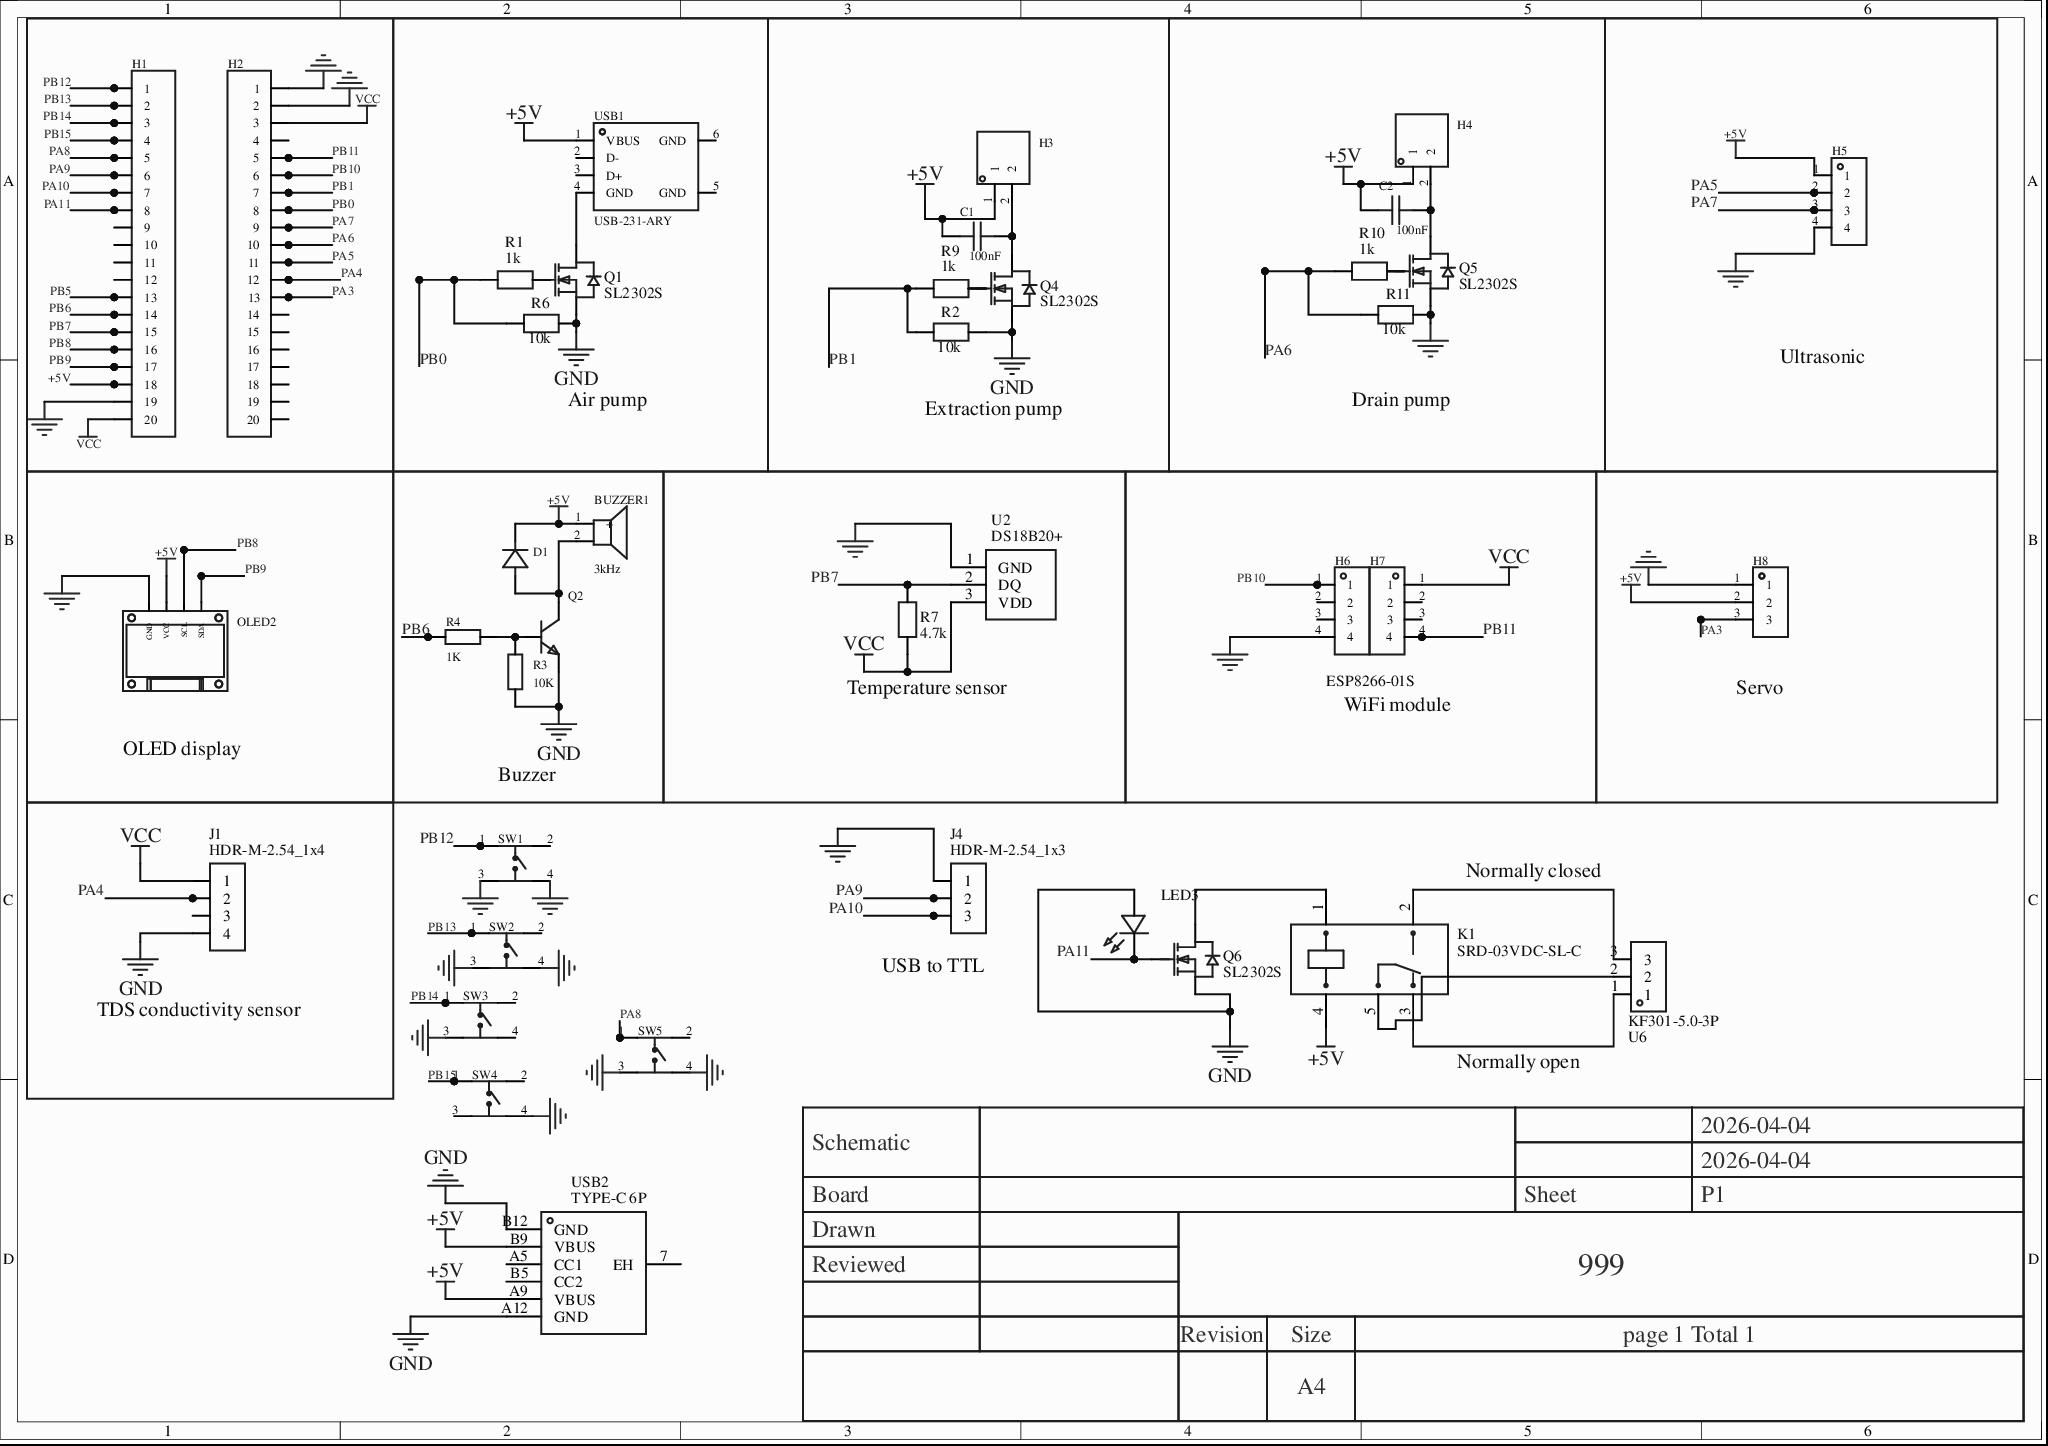
[diagram p0: MISC75408-3.schdoc]
# Altium project MISC75408-2.PrjPcb
1 sheet, 40 parts. Net scope: global (net labels, ports and power ports of the same name join across sheets).
Board file: MISC75408.pcbdoc

## Sheet MISC75408-3.schdoc
size 297 x 209 mm; Version: V1.0; @Project Name: MISC75408; @Update Date: 2026-04-16; @Create Date: 2026-04-16; @Board Name: MISC75408; @Create Time: 13:37:19; @Page Count: 1; @Page No: 1; @Schematic Name: MISC75408; @Update Time: 13:37:19; Size: A4

### Parts
BUZZER1  3kHz  [BUZ-TH_BD9.6-P5.00-D0.7-FD]
C1  100nF  [C0805]
C2  100nF  [C0805]
D1  (no value)  [DO_1N4007]
H1  (no value)  [HDR-TH_20P-P2.54-V-F]
H2  (no value)  [HDR-TH_20P-P2.54-V-F]
H3  (no value)  [HDR-TH_2P-P2.54-V-M-1]
H4  (no value)  [HDR-TH_2P-P2.54-V-M-1]
H5  (no value)  [HDR-TH_4P-P2.54-V-M]
H6  (no value)  [HDR-TH_4P-P2.54-V-M]
H7  (no value)  [HDR-TH_4P-P2.54-V-M]
H8  (no value)  [HDR-TH_3P-P2.54-V-M]
J1  HDR-M-2.54_1x4  [HDR-M-2.54_1X4]
J4  HDR-M-2.54_1x3  [HDR-M-2.54_1X3]
K1  SRD-03VDC-SL-C  [RELAY-TH_SRD-XXVDC-XL-C]
LED3  LED-TH-5mm_R  [LED-TH_BD5.0_RED]  (value not drawn)
OLED2  (no value)  [0.96OLED_4P]
Q1  SL2302S  [SOT-23_L2.9-W1.3-P1.90-LS2.4-BR]
Q2  (no value)  [S8050_TO_92]
Q4  SL2302S  [SOT-23_L2.9-W1.3-P1.90-LS2.4-BR]
Q5  SL2302S  [SOT-23_L2.9-W1.3-P1.90-LS2.4-BR]
Q6  SL2302S  [SOT-23_L2.9-W1.3-P1.90-LS2.4-BR]
R1  1k  [R0603]
R2  10k  [R0603]
R3  10K  [R0603]
R4  1K  [R0603]
R6  10k  [R0603]
R7  4.7k  [R0603]
R9  1k  [R0603]
R10  1k  [R0603]
R11  10k  [R0603]
SW1  J1L0503110  [SW-TH_4P-L6.0-W6.0-P4.50-LS6.3]  (value not drawn)
SW2  J1L0503110  [SW-TH_4P-L6.0-W6.0-P4.50-LS6.3]  (value not drawn)
SW3  J1L0503110  [SW-TH_4P-L6.0-W6.0-P4.50-LS6.3]  (value not drawn)
SW4  J1L0503110  [SW-TH_4P-L6.0-W6.0-P4.50-LS6.3]  (value not drawn)
SW5  J1L0503110  [SW-TH_4P-L6.0-W6.0-P4.50-LS6.3]  (value not drawn)
U2  DS18B20+  [HDR-TH_3P-P2.54-V-F]
U6  KF301-5.0-3P  [CONN-TH_3P-P5.00_KF301-5.0-3P]
USB1  USB-231-ARY  [USB-A-TH_USB-231-ARY]
USB2  TYPE-C 6P  [TYPE-C-SMD_TYPE-C-6P_1]

### Blocks framed on the sheet
Air pump: Q1 R1 R6 USB1
Extraction pump: C1 H3 Q4 R2 R9
Drain pump: C2 H4 Q5 R10 R11
Ultrasonic: H5
OLED display: OLED2
Buzzer: BUZZER1 D1 Q2 R3 R4
Temperature sensor: R7 U2
WiFi module: H6 H7
Servo: H8
TDS conductivity sensor: J1

### Nets
+5V: BUZZER1.1(+) C1.1 C2.1 D1.1(K) H1.18 H3.1 H4.1 H5.1 H8.2 K1.4 OLED2.2(VCC) USB1.1(VBUS) USB2.A9(VBUS) USB2.B9(VBUS)
GND: H1.19 H2.1 H2.2 H5.4 H6.4 H8.1 J1.4 J4.1 LED3.1 OLED2.1(GND) Q1.2(S) Q2.1(E) Q4.2(S) Q5.2(S) Q6.2(S) R2.2 R3.1 R6.2 R11.2 SW1.3 SW1.4 SW2.3 SW2.4 SW3.3 SW4.4 SW5.3 SW5.4 U2.1(GND) USB2.A12(GND) USB2.B12(GND)
VCC: H1.20 H2.3 H7.1 J1.1 R7.2 U2.3(VDD)
PA3: H2.13 H8.3
PA4: H2.12 J1.2
PA5: H2.11 H5.2
PA6: H2.10 R10.1 R11.1
PA7: H2.9 H5.3
PA8: H1.5 SW5.1
PA9: H1.6 J4.2
PA10: H1.7 J4.3
PA11: H1.8 LED3.2 Q6.1(G)
PB0: H2.8 R1.1 R6.1
PB1: H2.7 R2.1 R9.1
PB5: H1.13
PB6: H1.14 R4.2
PB7: H1.15 R7.1 U2.2(DQ)
PB8: H1.16 OLED2.3(SCL)
PB9: H1.17 OLED2.4(SDA)
PB10: H2.6 H6.1
PB11: H2.5 H7.4
PB12: H1.1 SW1.1
PB13: H1.2 SW2.1
PB14: H1.3 SW3.1
PB15: H1.4 SW4.1
NetBUZZER1_2: BUZZER1.2 D1.2(A) Q2.3(C)
NetC1_2: C1.2 H3.2 Q4.3(D)
NetC2_2: C2.2 H4.2 Q5.3(D)
NetK1_1: K1.1 Q6.3(D)
NetK1_2: K1.2 U6.3
NetK1_3: K1.3 U6.1
NetK1_5: K1.5 U6.2
NetQ1_1: Q1.1(G) R1.2
NetQ1_3: Q1.3(D) USB1.4(GND)
NetQ2_2: Q2.2(B) R3.2 R4.1
NetQ4_1: Q4.1(G) R9.2
NetQ5_1: Q5.1(G) R10.2

Not connected (* = marked no-connect by the designer): H1 9 10 11 12; H2 4 14 15 16 17 18 19 20; H6 2* 3*; H7 2* 3*; J1 3*; SW1 2*; SW2 2*; SW3 2* 4*; SW4 2* 3*; SW5 2*; USB1 2(D-)* 3(D+)* 5(GND)* 6(GND)*; USB2 7(EH)* A5(CC1)* B5(CC2)*

### Notes on the sheet
- ESP8266-01S
- Normally closed
- (near J4) USB to TTL
- Normally open
- 2026-04-04
- Schematic
- Board
- Sheet
- P1
- Drawn
- Reviewed
- 999
- Revision
- Size
- A4
- page 1 Total 1

### Library data of the parts
BUZZER1 = HNB09A05: Drive method: active (built-in driver circuit); Construction type: electromagnetic; Rated voltage: -; Frequency: 3kHz; Sound pressure (SPL): 85dB;; Manufacturer: 华能; 3D Model: 13273335caac486e928bafb4d9fdf12d0819f05c4eef4c71ace90d822a990e87; 3D Model Transform: 354.33,354.33,0,90,0,0,0,0,-177.165; Voltage - Supply: 3V~7V; AddInBom: yes; ModelName: BUZ-TH_D9.0-H5.5-P5.0; Device: HNB09A05; Symbol: HNB09A05; LCSC Part Name: HNB09A05; Supplier Part: C96493; Manufacturer Part: HNB09A05; Supplier Footprint: 插件,D=9mm; JLCPCB Part Class: Extended Part; Datasheet: https://example.com/datasheet/HNB09A05/97698.html; Supplier: LCSC; Driver Circuitry: Active (built-in driver circuit); Technology: Electromagnetic; Voltage Rating: -; Value: 3kHz; Current Consumption: -; Sound Pressure Level(SPL): 85dB; Diameter(φD): 9mm; Length: -; Width: -; Height: 5.7mm; Operating Temperature: -; FootprintName: BUZ-TH_BD9.6-P5.00-D0.7-FD; ConvertToPcb: yes
C1 C2 = CAP_0805: Symbol: Capacitance; ConvertToPcb: yes; ModelId: 1ba041120af144c991958decab20d2410819f05c4eef4c71ace90d822a990e87; ModelName: C0805_L2.0-W1.3-H1.3; ModelTransform: 78.74,51.181,0,0,0,0,0,0.0005,0; Device: CAP_0805; FootprintName: C0805; AddInBom: yes; Supplier Footprint: 0805; Value: 100nF
D1 = D_1N4007A: AddInBom: yes; ModelId: 6de1e9b71a0d4751b4e9df530304c1a30819f05c4eef4c71ace90d822a990e87; ModelName: DO-41_D2.4-L4.7-P8.70; ModelTransform: 373.9,94.4,232.29,0,0,0,0,0,-140; Device: D_1N4007A; Symbol: D_1N4007; FootprintName: DO_1N4007; Supplier Footprint: DO-41; ConvertToPcb: yes
H1 H2 = HDR-F_2.54_1x20P: 3D Model: db7015f7ad9d48b8a3b1188db02e34290819f05c4eef4c71ace90d822a990e87; 3D Model Transform: 1999.996,100,0,0,0,0,0,0,-118.11; ConvertToPcb: yes; ModelName: HDR-F-2.54_1x20; Device: HDR-F_2.54_1x20P; Symbol: HDR-F_2.54_1x20P; Supplier Part: C50984; Supplier Footprint: 插件; FootprintName: HDR-TH_20P-P2.54-V-F; AddInBom: yes
H3 H4 = HDR-M_2.54_1x2P: Symbol: 210S-1*2P L=11.6MMGold-plated black; ConvertToPcb: yes; ModelId: 79b2e9f2d70a4d68a1b7098f27c6d4c50819f05c4eef4c71ace90d822a990e87; ModelName: HDR-M-2.54_1x2; ModelTransform: 200,100,0,0,0,0,0,0,-118.11; Device: HDR-M_2.54_1x2P; FootprintName: HDR-TH_2P-P2.54-V-M-1; AddInBom: yes; SupplierPart: C124375; Supplier Footprint: 插件
H5-H7 = HDR-M_2.54_1x4P: Symbol: PZ254V-11-04P; ConvertToPcb: yes; ModelId: 112f4d05e8d64e99ab9a333894bea4f90819f05c4eef4c71ace90d822a990e87; ModelName: HDR-TH_4P-P2.54-M-LI-1X4P; ModelTransform: 399.999,104.7242,0,0,0,0,0,0,-118.11; Device: HDR-M_2.54_1x4P; FootprintName: HDR-TH_4P-P2.54-V-M; AddInBom: yes; SupplierPart: C492403; Supplier Footprint: 插件
H8 = HDR-M_2.54_1x3P: AddInBom: yes; ModelId: bb473b6d38ff42a99216a4fcdbdcc4cb0819f05c4eef4c71ace90d822a990e87; ModelName: HDR-TH_3P-P2.54-M-LI-1X3P; ModelTransform: 300.03877,100,0,0,0,0,0,0,-118.11; Device: HDR-M_2.54_1x3P; Symbol: HDR-M_2.54_1x3P; FootprintName: HDR-TH_3P-P2.54-V-M; ConvertToPcb: yes; SupplierPart: C2937625; Supplier Footprint: 插件
J1 = HDR-M-2.54_1x4: Add into BOM: yes; ModelId: cd502121c3eb48dbbf0ecbc8e7ad097f; ModelTransform: 0,0,0,0,0,0,0,0,0; Device: HDR-M-2.54_1x4; Symbol: HDR-M-2.54_1x4; Convert to PCB: yes; Supplier Part: C124378; Supplier: LCSC; Origin 3D Model Title: HDR-M-2.54_1X4; FootprintName: HDR-M-2.54_1X4; ModelName: HDR-M-2.54_1X4
J4 = HDR-M-2.54_1x3: Add into BOM: yes; ModelId: e45037aab22c4927a5ea885f2a5b96c9; ModelTransform: 0,0,0,0,0,0,0,0,0; Device: HDR-M-2.54_1x3; Symbol: HDR-M-2.54_1x3; Convert to PCB: yes; Supplier Part: C180248; Supplier: LCSC; Origin 3D Model Title: HDR-M-2.54_1x3; FootprintName: HDR-M-2.54_1X3; ModelName: HDR-M-2.54_1x3
K1 = SRD-03VDC-SL-C: Manufacturer: 松乐; Add into BOM: yes; Origin 3D Model Title: RELAY-TH_L19.2-W15.6-H15.8; ModelId: d0eda9b8bf8746d18ae810ab88dc78e7; ModelTransform: 0,0,0,0,0,0,0,0,0; Device: SRD-03VDC-SL-C; Symbol: SRD-03VDC-SL-C; Convert to PCB: yes; Supplier: LCSC; Manufacturer Part: SRD-03VDC-SL-C; Supplier Part: C24585; JLCPCB Part Class: Extended Part; FootprintName: RELAY-TH_SRD-XXVDC-XL-C; ModelName: RELAY-TH_L19.2-W15.6-H15.8
LED3 = LED-TH-5mm_R: Manufacturer: EVERLIGHT(台湾亿光); Manufacturer Part: 333-2SURD/S530-A3; Add into BOM: yes; ModelId: 0e3e1c3f5c0d4d279dc0d0ab1929e6bc; ModelTransform: 0,0,0,0,0,0,0,0,0; Device: LED-TH-5mm_R; Symbol: LED-TH-5mm_R; Convert to PCB: yes; Supplier Part: C87271; Supplier: LCSC; Origin 3D Model Title: LED-TH_BD5.0_Red; FootprintName: LED-TH_BD5.0_RED; ModelName: LED-TH_BD5.0_Red
OLED2 = 0.96OLED模块_4P: Device: 0.96OLED module_4P; ConvertToPcb: yes; ModelId: 79c000fdb68d45a296c2e9bedf4f90550819f05c4eef4c71ace90d822a990e87; ModelTransform: 1393.69792,1318.895,0,0,0,0,0,-560.079,-137.795; Symbol: 0.96OLED module_4P; FootprintName: 0.96OLED_4P; AddInBom: yes; Supplier Footprint: 插件; ModelName: 0.96OLED_4P
Q1 Q4-Q6 = SL2302S: Manufacturer: Slkor(萨科微); Add into BOM: yes; Origin 3D Model Title: SOT-23-3P_L2.9-W1.3-H1.0-LS2.4-P0.95; ModelId: c62791f0466c4ae2a892c056b845b0ca; ModelTransform: 0,0,0,0,0,0,0,0,0; Device: SL2302S; Symbol: SL2302S; Convert to PCB: yes; Supplier: LCSC; Supplier Part: C473811; Manufacturer Part: SL2302S; JLCPCB Part Class: Extended Part; FootprintName: SOT-23_L2.9-W1.3-P1.90-LS2.4-BR; ModelName: SOT-23-3P_L2.9-W1.3-H1.0-LS2.4-P0.95
Q2 = S8050_TO_NPN: ConvertToPcb: yes; ModelId: aafe8e06f2154e7c93506efd0d6632dd0819f05c4eef4c71ace90d822a990e87; ModelName: TO-92-3_L4.9-W3.7-P1.27-L; ModelTransform: 180.78,141.44,417.3,0,0,0,0,0,-200; Device: S8050_TO_NPN; Symbol: S8050_TO_NPN; FootprintName: S8050_TO_92; AddInBom: yes; Supplier Footprint: TO-92
R1 R9 R10 = 1k: Add into BOM: yes; ModelId: fc143cca1e79419f9cd78b61e9279f08; ModelTransform: 0,0,0,0,0,0,0,0,0; Device: 1k; Symbol: 1k; Convert to PCB: yes; Origin 3D Model Title: R0603; FootprintName: R0603; ModelName: R0603
R2 R6 R7 R11 = 10k: Add into BOM: yes; ModelId: fc143cca1e79419f9cd78b61e9279f08; ModelTransform: 0,0,0,0,0,0,0,0,0; Device: 10k; Symbol: 10k; Convert to PCB: yes; Origin 3D Model Title: R0603; FootprintName: R0603; ModelName: R0603
R3 R4 = Res_0603: Symbol: Resistor; ConvertToPcb: yes; ModelId: fc143cca1e79419f9cd78b61e9279f080819f05c4eef4c71ace90d822a990e87; ModelTransform: 31.8897,63.7794,0,90,0,0,0,0,0; Device: Res_0603; FootprintName: R0603; AddInBom: yes; Supplier Footprint: 0603; ModelName: R0603
  R3: Value: 10K
  R4: Value: 1K
SW1-SW5 = J1L0503110: Circuit structure: SPST; Button shape: round button; Actuating force: 2.6N; Mounting: through-hole; Switch length: 6mm; Switch width: 6mm; Switch height: 5mm; With bracket: -; Contact current: 50mA; Rated voltage: 12V; With lamp: none; Operating life: 10万 cycles;; Manufacturer: SAMZO(三佐); 3D Model: f12d4fb4f8314a3f92db4aebb329b4320819f05c4eef4c71ace90d822a990e87; 3D Model Transform: 306.99781,236.22,0,0,0,0,0,0,-137.795; Actuator/Cap Color: Black; AddInBom: yes; Device: J1L0503110; Symbol: J1L0503110; LCSC Part Name: 6*6*5 四脚插件 铜盖 260gf; Supplier Part: C29780808; Manufacturer Part: J1L0503110; Supplier Footprint: 插件-4P,6x6mm; JLCPCB Part Class: Extended Part; Datasheet: https://example.com/datasheet/J1L0503110/31512971.html; Supplier: LCSC; Circuit: SPST; Actuator Style: Round button; Operating Force: 2.6N; Mounting Type: Through-hole; Length: 6mm; Width: 6mm; Switch Height: 5mm; with Bracket: -; Contact Current: 50mA; Voltage Rating: 12V; With Lamp: None; IP Rating: -; Termination Style: -; Life: 10万 cycles; Operating Temperature: -25℃~+85℃; FootprintName: SW-TH_4P-L6.0-W6.0-P4.50-LS6.3; ConvertToPcb: yes; ModelName: SW-TH_4P-L6.0-W6.0-P4.50-LS6.3
U2 = DS18B20+: Manufacturer: ADI(亚德诺)/MAXIM(美信); Add into BOM: yes; Origin 3D Model Title: TO-92-3_L4.9-W3.7-P1.27-L; ModelId: aafe8e06f2154e7c93506efd0d6632dd; ModelTransform: 0,0,0,0,0,0,0,0,0; Device: DS18B20+; Symbol: DS18B20+; Convert to PCB: yes; Supplier: LCSC; Manufacturer Part: DS18B20+; Supplier Part: C9753; JLCPCB Part Class: Extended Part; FootprintName: HDR-TH_3P-P2.54-V-F; ModelName: TO-92-3_L4.9-W3.7-P1.27-L
U6 = KF301-5.0-3P: Manufacturer: KEFA(科发); Add into BOM: yes; ModelId: 7090fd1e13c24e5e88660dd73c452457; ModelTransform: 0,0,0,0,0,0,0,0,0; Device: KF301-5.0-3P; Symbol: KF301-5.0-3P; Convert to PCB: yes; Supplier: LCSC; Supplier Part: C474882; Manufacturer Part: KF301-5.0-3P; JLCPCB Part Class: Extended Part; Origin 3D Model Title: CONN-TH_3P-P5.00_KF301-5.0-3P; FootprintName: CONN-TH_3P-P5.00_KF301-5.0-3P; ModelName: CONN-TH_3P-P5.00_KF301-5.0-3P
USB1 = USB-231-ARY: Connector type: Type-A; Protocol standard: USB 2.0; Gender: female; Mounting: right angle; Contacts: 4P; Ports: 1; Rated current - power: 1.5A; Operating temperature: -20℃~+70℃;; Manufacturer: XUNPU(讯普); AddInBom: yes; Protocol Standard: USB 2.0; Number of Ports: 1; Voltage Rating: 30V; Detection color: White; ModelId: 2c22904cfa634797a8992a7288a8f2530819f05c4eef4c71ace90d822a990e87; ModelTransform: 610.18209,551.18,0,0,0,0,0,-183.071,-137.795; Device: USB-231-ARY; Symbol: USB-231-ARY; FootprintName: USB-A-TH_USB-231-ARY; LCSC Part Name: Type-A 母 弯插; SupplierPart: C720525; ManufacturerPart: USB-231-ARY; Supplier Footprint: 弯插; JLCPCB Part Class: Extended Part; Datasheet: https://example.com/datasheet/USB-231-ARY/763532.html; Supplier: LCSC; ConvertToPcb: yes; Connector Type: Type-A; Gender: Female; Mounting Type: Right angle; Number of Contacts: 4P; Current Rating-Power: 1.5A; Length: 14.2mm; Operating Temperature: -20℃~+70℃; ModelName: USB-A-TH_USB-231-ARY
USB2 = TYPE-C 6P: Manufacturer: SHOU HAN(首韩); Add into BOM: yes; Origin 3D Model Title: TYPE-C-SMD_6P-L8.9-W6.8-H3.2-P1.00; ModelId: 3770c5585474407db939b2377e27177a; ModelTransform: 0,0,0,0,0,0,0,0,0; Device: TYPE-C 6P; Symbol: TYPE-C 6P; Convert to PCB: yes; Supplier: LCSC; Supplier Part: C456012; Manufacturer Part: TYPE-C 6P; JLCPCB Part Class: Extended Part; FootprintName: TYPE-C-SMD_TYPE-C-6P_1; ModelName: TYPE-C-SMD_6P-L8.9-W6.8-H3.2-P1.00